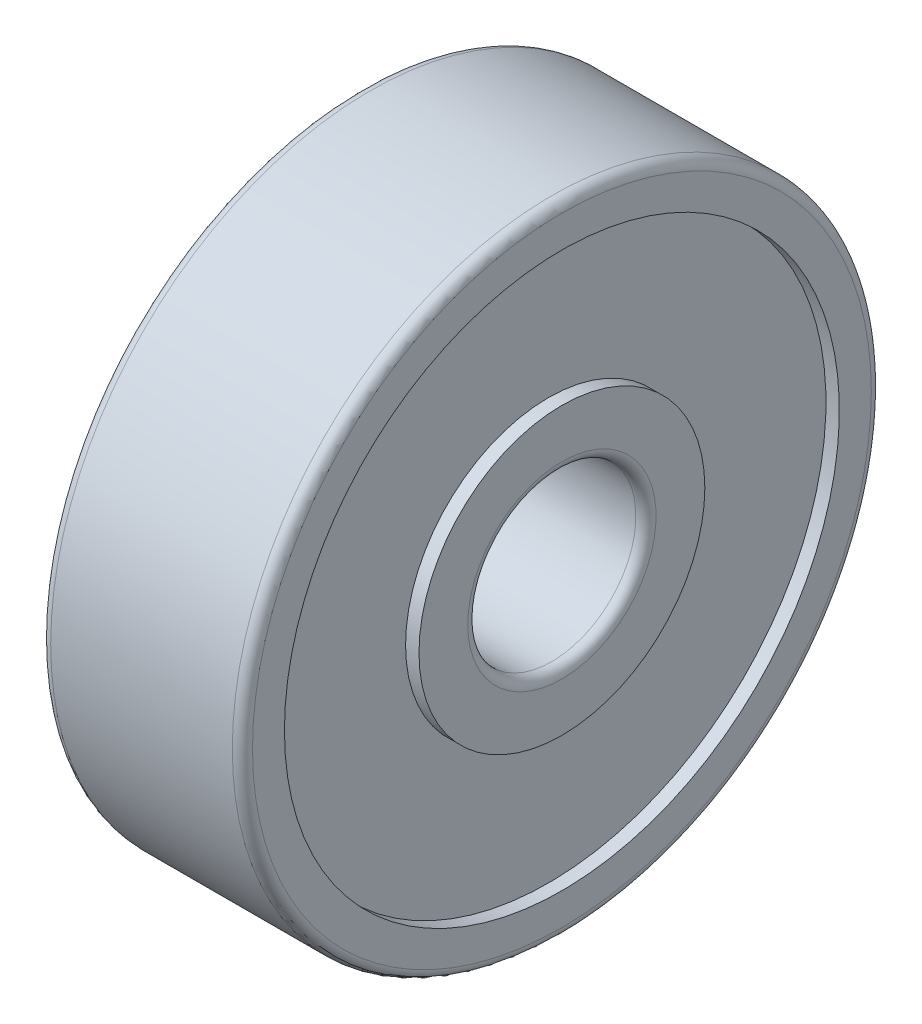
from build123d import *


with BuildPart() as part:
    # 草图1 → 旋转1 (revolve)
    with BuildSketch(Plane.XY, mode=Mode.PRIVATE) as revolve_1_sk:
        with BuildLine():
            Line((0, 9.2), (0, 8.25))
            Line((0, 8.25), (0.3984, 8.25))
            Line((0.3984, 8.25), (0.3984, 4.25))
            Line((0.3984, 4.25), (0, 4.25))
            Line((0, 4.25), (0, 2.8))
            ThreePointArc((0, 2.8), (0.087867966, 2.587867966), (0.3, 2.5))
            Line((0.3, 2.5), (5.7, 2.5))
            ThreePointArc((5.7, 2.5), (5.912132034, 2.587867966), (6, 2.8))
            Line((6, 2.8), (6, 4.25))
            Line((6, 4.25), (5.6016, 4.25))
            Line((5.6016, 4.25), (5.6016, 8.25))
            Line((5.6016, 8.25), (6, 8.25))
            Line((6, 8.25), (6, 9.2))
            ThreePointArc((6, 9.2), (5.912132034, 9.412132034), (5.7, 9.5))
            Line((5.7, 9.5), (0.3, 9.5))
            ThreePointArc((0.3, 9.5), (0.087867966, 9.412132034), (0, 9.2))
        make_face()
    revolve(revolve_1_sk.sketch.rotate(Axis((5.7, 0, 0), (-1, 0, 0)), 270), axis=Axis((5.7, 0, 0), (-1, 0, 0)))


solid = part.part
